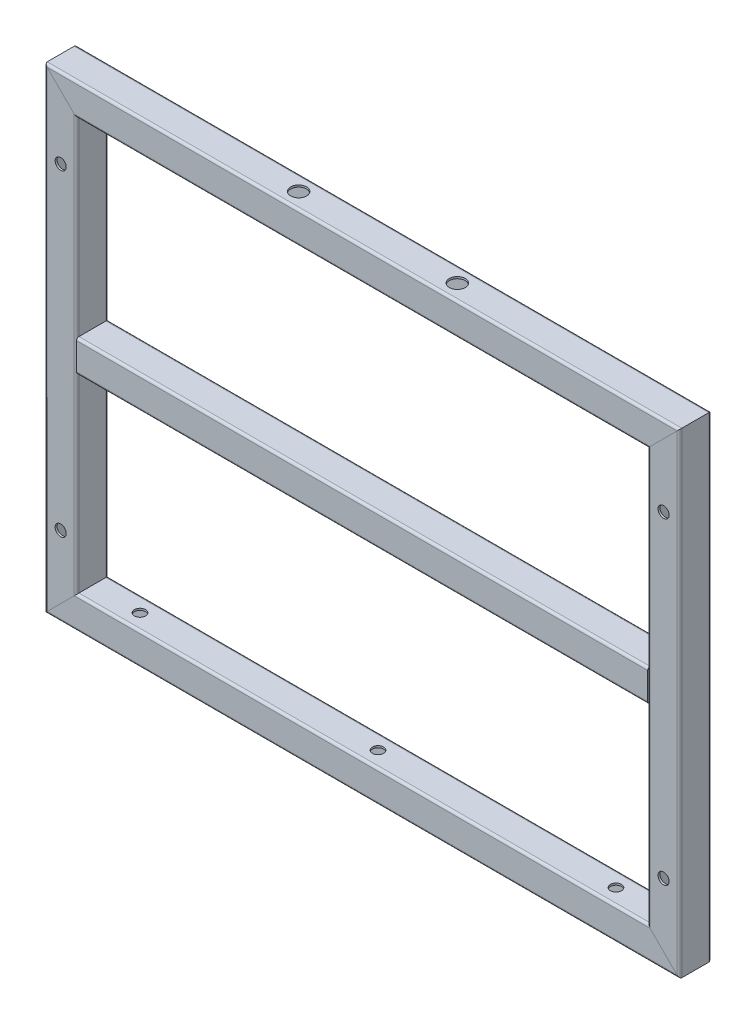
SolidWorks part; units mm, degrees
ref_plane "Front Plane" through (0, 0, 0) normal (0, 0, 1) x (1, 0, 0)
ref_plane "Top Plane" through (0, 0, 0) normal (0, 1, 0) x (1, 0, 0)
ref_plane "Right Plane" through (0, 0, 0) normal (1, 0, 0) x (0, 0, -1)
sketch "草图1" plane through (0, 0, 0) normal (0, 0, 1) x (1, 0, 0)
  line L0 (-190, 0) -> (190, 0)
  line L1 (190, 140) -> (-190, 140)
  line L2 (190, 140) -> (190, -140)
  line L3 (190, -140) -> (-190, -140)
  line L4 (-190, 140) -> (-190, -140)
  line L5 (190, 140) -> (-190, -140) construction
  line L6 (190, -140) -> (-190, 140) construction
  point P0 (0, 0)
  dimension "D1" = 380
  dimension "D2" = 280
other "Structural Member1"
ref_plane "Plane1" through (190, 140, 0) normal (-1, 0, 0) x (0, -1, 0)
sketch "Sketch1" plane through (190, 140, 0) normal (-1, 0, 0) x (0, -1, 0)
  line L0 (-8.5, -8.8) -> (8.5, -8.8)
  line L1 (-8.8, -8.5) -> (-8.8, 8.5)
  line L2 (8.5, 8.8) -> (-8.5, 8.8)
  line L3 (8.8, 8.5) -> (8.8, -8.5)
  line L4 (-8.5, -10) -> (8.5, -10)
  line L5 (-10, -8.5) -> (-10, 8.5)
  line L6 (8.5, 10) -> (-8.5, 10)
  line L7 (10, 8.5) -> (10, -8.5)
  arc A0 (10, 8.5) -> (8.5, 10) centre (8.5, 8.5) ccw
  arc A1 (8.5, -10) -> (10, -8.5) centre (8.5, -8.5) ccw
  arc A2 (-10, -8.5) -> (-8.5, -10) centre (-8.5, -8.5) ccw
  arc A3 (-8.5, 10) -> (-10, 8.5) centre (-8.5, 8.5) ccw
  arc A4 (-8.5, 8.8) -> (-8.8, 8.5) centre (-8.5, 8.5) ccw
  arc A5 (8.8, 8.5) -> (8.5, 8.8) centre (8.5, 8.5) ccw
  arc A6 (8.5, -8.8) -> (8.8, -8.5) centre (8.5, -8.5) ccw
  arc A7 (-8.8, -8.5) -> (-8.5, -8.8) centre (-8.5, -8.5) ccw
  point P0 (-10, 0)
  point P1 (10, 0)
  point P2 (0, 10)
  point P3 (0, -10)
  point P4 (0, 0)
  point P5 (-10, -10)
  point P6 (10, -10)
  point P7 (10, 10)
  point P8 (-10, 10)
  point P33 (0, 0)
  dimension "D1" = 1.5
  dimension "Thickness" = 1.2
  dimension "V_leg" = 20
sketch "Sketch3" plane through (0, 0, 10) normal (0, 0, 1) x (1, 0, 0)
  line L0 (-200, -150) -> (-200, 150) construction
  line L1 (-198.5, -148.5) -> (-198.5, 148.5) construction
  line L2 (0, 131.5) -> (0, -148.5) construction
  line L3 (-181.5, 131.5) -> (181.5, 131.5) construction
  line L4 (198.5, -148.5) -> (-198.5, -148.5) construction
  line L5 (-198.5, 0) -> (198.5, 0) construction
  line L6 (198.5, 148.5) -> (198.5, -148.5) construction
  circle A0 centre (-190, 100) radius 3.5
  circle A1 centre (-190, -100) radius 3.5
  circle A2 centre (190, -100) radius 3.5
  circle A3 centre (190, 100) radius 3.5
  point P4 (-198.5, 0)
  dimension "D1" = 10
  dimension "D2" = 100
extrude "Cut-Extrude1" cut sketch "Sketch3" against normal through all
sketch "Sketch4" plane through (0, 150, 0) normal (0, 1, 0) x (-1, 0, 0)
  line L0 (200, 8.5) -> (-200, 8.5) construction
  circle A0 centre (50, 0) radius 5
  circle A1 centre (-50, 0) radius 5
  point P4 (0, 8.5)
  dimension "D1" = 100
  dimension "D2" = 50
extrude "Cut-Extrude2" cut sketch "Sketch4" against normal blind 10
sketch "Sketch5" plane through (0, -130, 0) normal (0, 1, 0) x (-1, 0, 0)
  line L0 (-180, 8.5) -> (180, 8.5) construction
  circle A0 centre (0, 0) radius 3.5
  circle A1 centre (-150, 0) radius 3.5
  circle A2 centre (150, 0) radius 3.5
  point P6 (0, 8.5)
  dimension "D1" = 150
  dimension "D2" = 0
  dimension "D3" = 150
extrude "Cut-Extrude3" cut sketch "Sketch5" against normal blind 20
